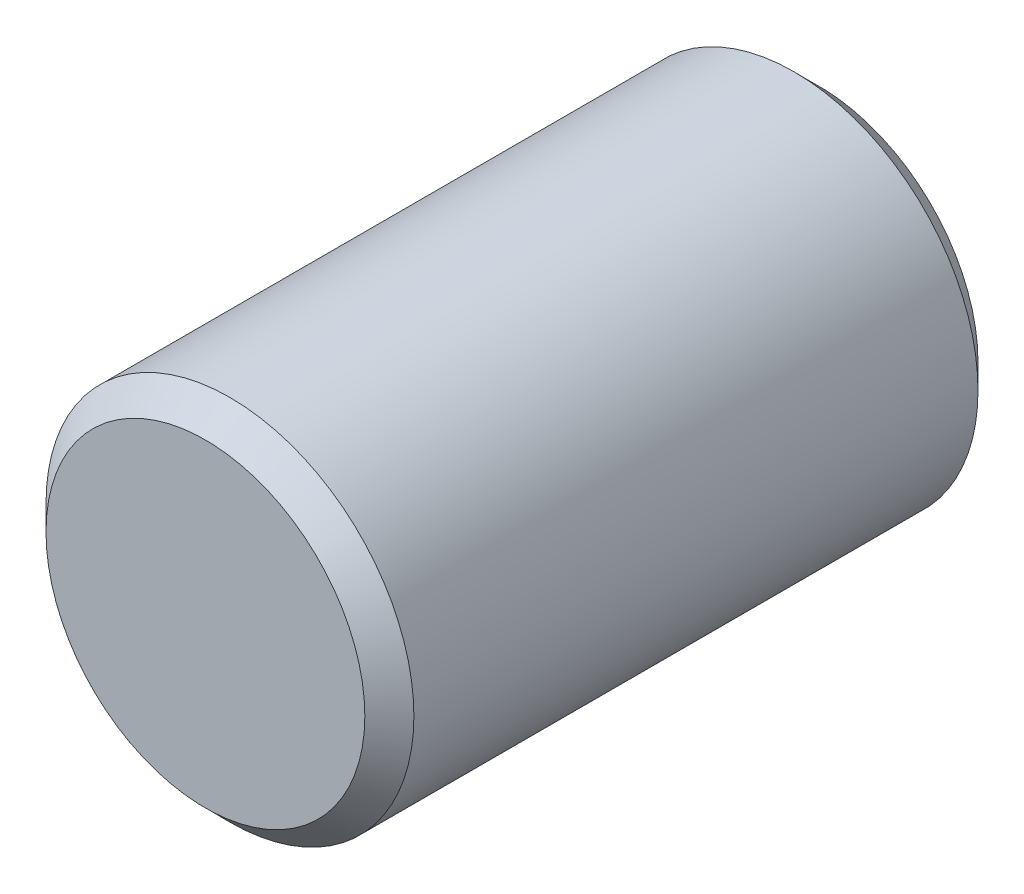
from build123d import *

# Parameters (mm, degrees)
SKETCH1_R           = 1.5
BOSS_EXTRUDE1_DEPTH = 5
CHAMFER1_SIZE       = 0.2


with BuildPart() as part:
    # Sketch1 → Boss-Extrude1 (new body)
    with BuildSketch(Plane.XY):
        Circle(SKETCH1_R)
    extrude(amount=BOSS_EXTRUDE1_DEPTH)

    # Chamfer1
    chamfer1_edges = [part.edges().sort_by_distance(p)[0] for p in [
        (-1.5, 0, 0),
        (-1.5, 0, 5),
    ]]
    chamfer(chamfer1_edges, length=CHAMFER1_SIZE)


solid = part.part
